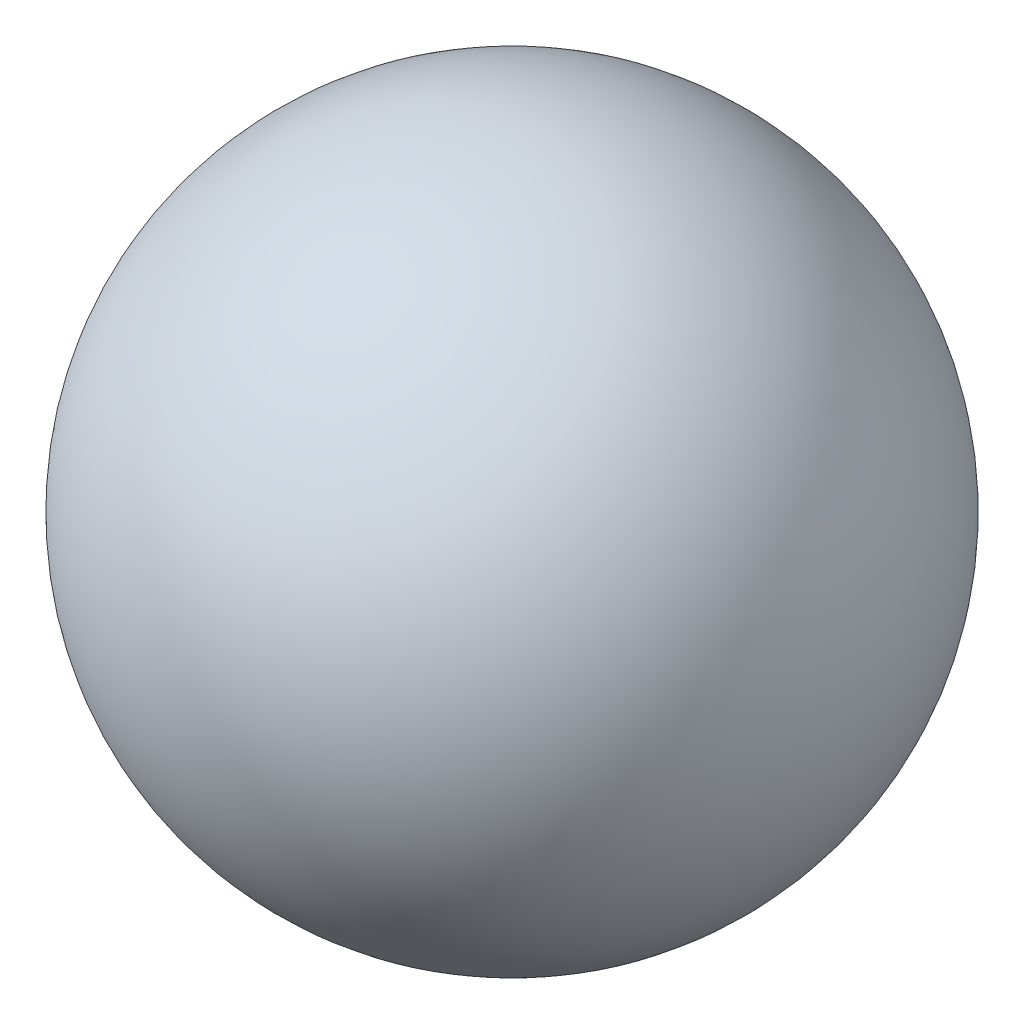
SolidWorks part; units mm, degrees
ref_plane "前视基准面" through (0, 0, 0) normal (0, 0, 1) x (1, 0, 0)
ref_plane "上视基准面" through (0, 0, 0) normal (0, 1, 0) x (1, 0, 0)
ref_plane "右视基准面" through (0, 0, 0) normal (1, 0, 0) x (0, 0, -1)
sketch "草图1" plane through (0, 0, 0) normal (0, 0, 1) x (1, 0, 0)
  line L0 (0, 25) -> (0, -25)
  arc A0 (0, -25) -> (0, 25) centre (0, 0) ccw
  dimension "D1" = 25
revolve "旋转1" add sketch "草图1" angle 360 about L0
